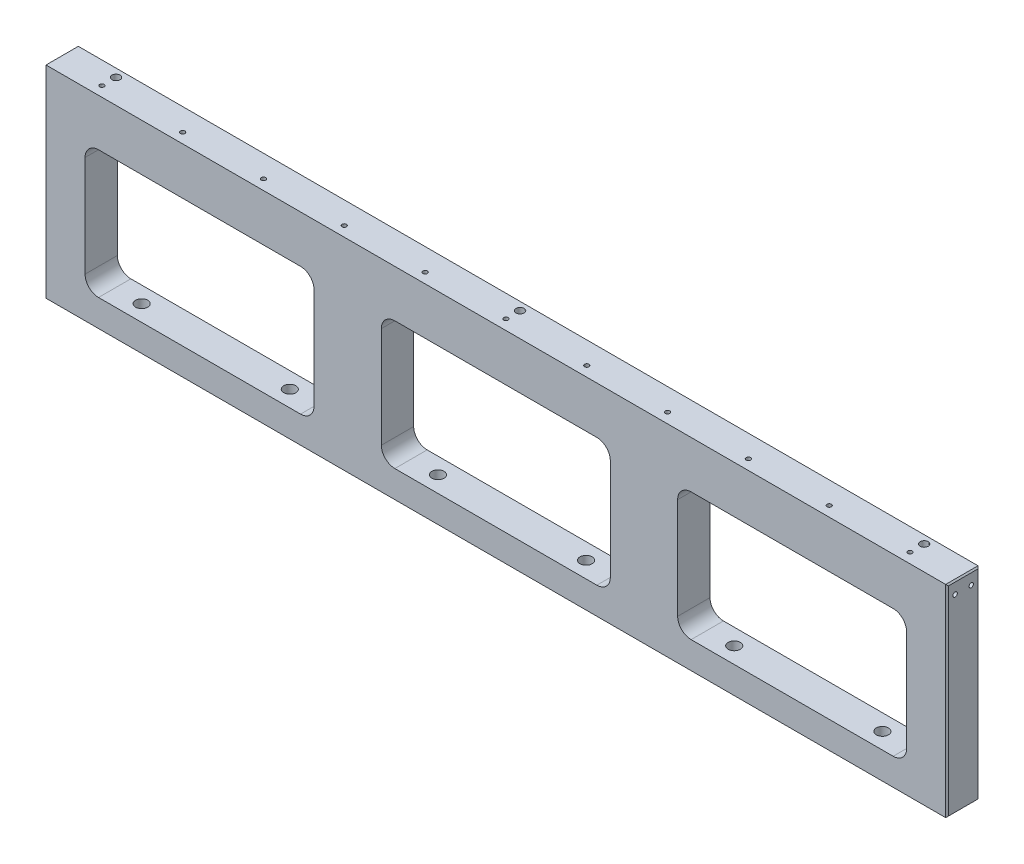
from build123d import *

# Parameters (mm, degrees)
SKETCH1_W                     = 670
SKETCH1_H                     = 150
BOSS_EXTRUDE1_DEPTH           = 12
CUT_EXTRUDE1_DEPTH            = 345.13078909
M8_CLEARANCE_HOLE1_D          = 9
M8_CLEARANCE_HOLE1_DEPTH      = 20
M4_TAPPED_HOLE1_D             = 3.3
M4_TAPPED_HOLE1_DEPTH         = 10.1
M4_TAPPED_HOLE1_TIP           = 0.991420021
SIZE_MM_BLIND_PIN_HOLE1_D     = 6
SIZE_MM_BLIND_PIN_HOLE1_DEPTH = 10.1
SIZE_MM_BLIND_PIN_HOLE1_TIP   = 1.802581857
CHAMFER1_SIZE                 = 1
M4_TAPPED_HOLE2_D             = 3.3
M4_TAPPED_HOLE2_DEPTH         = 10.1
M4_TAPPED_HOLE2_TIP           = 0.991420021
M4_TAPPED_HOLE3_D             = 3.3
M4_TAPPED_HOLE3_DEPTH         = 10.1
M4_TAPPED_HOLE3_TIP           = 0.991420021
M3_TAPPED_HOLE1_D             = 2.5
M3_TAPPED_HOLE1_DEPTH         = 7.5
M3_TAPPED_HOLE1_TIP           = 0.751075774
M4_TAPPED_HOLE4_D             = 3.3
M4_TAPPED_HOLE4_DEPTH         = 10.1
M4_TAPPED_HOLE4_TIP           = 0.991420021


with BuildPart() as part:
    # Sketch1 → Boss-Extrude1 (new, symmetric)
    with BuildSketch(Plane.XY):
        Rectangle(SKETCH1_W, SKETCH1_H)
    extrude(amount=BOSS_EXTRUDE1_DEPTH, both=True)

    # Sketch2 → Cut-Extrude1 (cut, through all)
    with BuildSketch(Plane.XY.offset(12)):
        with BuildLine():
            Line((-295, 40), (-145, 40))
            ThreePointArc((-145, 40), (-137.928932188, 37.071067812), (-135, 30))
            Line((-135, 30), (-135, -45))
            ThreePointArc((-135, -45), (-137.928932188, -52.071067812), (-145, -55))
            Line((-145, -55), (-295, -55))
            ThreePointArc((-295, -55), (-302.071067812, -52.071067812), (-305, -45))
            Line((-305, -45), (-305, 30))
            ThreePointArc((-305, 30), (-302.071067812, 37.071067812), (-295, 40))
        make_face()
        with BuildLine():
            Line((-75, 40), (75, 40))
            ThreePointArc((75, 40), (82.071067812, 37.071067812), (85, 30))
            Line((85, 30), (85, -45))
            ThreePointArc((85, -45), (82.071067812, -52.071067812), (75, -55))
            Line((75, -55), (-75, -55))
            ThreePointArc((-75, -55), (-82.071067812, -52.071067812), (-85, -45))
            Line((-85, -45), (-85, 30))
            ThreePointArc((-85, 30), (-82.071067812, 37.071067812), (-75, 40))
        make_face()
        with BuildLine():
            Line((145, 40), (295, 40))
            ThreePointArc((295, 40), (302.071067812, 37.071067812), (305, 30))
            Line((305, 30), (305, -45))
            ThreePointArc((305, -45), (302.071067812, -52.071067812), (295, -55))
            Line((295, -55), (145, -55))
            ThreePointArc((145, -55), (137.928932188, -52.071067812), (135, -45))
            Line((135, -45), (135, 30))
            ThreePointArc((135, 30), (137.928932188, 37.071067812), (145, 40))
        make_face()
    extrude(amount=-CUT_EXTRUDE1_DEPTH, mode=Mode.SUBTRACT)

    # M8 Clearance Hole1
    with Locations(Plane(origin=(0, -75, 0), x_dir=(-1, 0, 0), z_dir=(0, -1, 0))):
        with Locations((-275, 0), (275, 0), (165, 0), (55, 0), (-55, 0), (-165, 0)):
            Hole(M8_CLEARANCE_HOLE1_D / 2, depth=M8_CLEARANCE_HOLE1_DEPTH)

    # M4 Tapped Hole1
    with Locations(Plane(origin=(0, 75, 0), x_dir=(1, 0, 0), z_dir=(0, 1, 0))):
        with Locations((-300, -4.5), (-240, -4.5), (-180, -4.5), (-120, -4.5), (-60, -4.5), (0, -4.5), (60, -4.5), (120, -4.5), (180, -4.5), (240, -4.5), (300, -4.5)):
            Hole(M4_TAPPED_HOLE1_D / 2, depth=M4_TAPPED_HOLE1_DEPTH)
            with Locations((0, 0, -(M4_TAPPED_HOLE1_DEPTH + M4_TAPPED_HOLE1_TIP / 2))):  # 118° drill point
                Cone(0, M4_TAPPED_HOLE1_D / 2, M4_TAPPED_HOLE1_TIP, mode=Mode.SUBTRACT)

    # Size mm Blind Pin Hole1
    with Locations(Plane(origin=(0, 75, 0), x_dir=(1, 0, 0), z_dir=(0, 1, 0))):
        with Locations((300, 6), (-300, 6), (0, 6)):
            Hole(SIZE_MM_BLIND_PIN_HOLE1_D / 2, depth=SIZE_MM_BLIND_PIN_HOLE1_DEPTH)
            with Locations((0, 0, -(SIZE_MM_BLIND_PIN_HOLE1_DEPTH + SIZE_MM_BLIND_PIN_HOLE1_TIP / 2))):  # 118° drill point
                Cone(0, SIZE_MM_BLIND_PIN_HOLE1_D / 2, SIZE_MM_BLIND_PIN_HOLE1_TIP, mode=Mode.SUBTRACT)

    # Chamfer1
    chamfer1_edges = [part.edges().sort_by_distance(p)[0] for p in [
        (-335, 0, 12),
        (335, 0, 12),
        (-335, 0, -12),
        (335, 0, -12),
        (335, -75, 0),
        (-335, -75, 0),
        (-335, 75, 0),
        (335, 75, 0),
    ]]
    chamfer(chamfer1_edges, length=CHAMFER1_SIZE)

    # M4 Tapped Hole2
    with Locations(Plane(origin=(335, 0, 0), x_dir=(0, 0, -1), z_dir=(1, 0, 0))):
        with Locations((6, 66), (-6, 66)):
            Hole(M4_TAPPED_HOLE2_D / 2, depth=M4_TAPPED_HOLE2_DEPTH)
            with Locations((0, 0, -(M4_TAPPED_HOLE2_DEPTH + M4_TAPPED_HOLE2_TIP / 2))):  # 118° drill point
                Cone(0, M4_TAPPED_HOLE2_D / 2, M4_TAPPED_HOLE2_TIP, mode=Mode.SUBTRACT)

    # M4 Tapped Hole3
    with Locations(Plane.ZY.offset(335)):
        with Locations((-6, 66), (6, 66)):
            Hole(M4_TAPPED_HOLE3_D / 2, depth=M4_TAPPED_HOLE3_DEPTH)
            with Locations((0, 0, -(M4_TAPPED_HOLE3_DEPTH + M4_TAPPED_HOLE3_TIP / 2))):  # 118° drill point
                Cone(0, M4_TAPPED_HOLE3_D / 2, M4_TAPPED_HOLE3_TIP, mode=Mode.SUBTRACT)

    # M3 Tapped Hole1
    with Locations(Plane(origin=(0, 0, -12), x_dir=(1, 0, 0), z_dir=(0, 0, -1))):
        with Locations((314.85, -59), (-314.85, -59), (-295.15, -59), (295.15, -59)):
            Hole(M3_TAPPED_HOLE1_D / 2, depth=M3_TAPPED_HOLE1_DEPTH)
            with Locations((0, 0, -(M3_TAPPED_HOLE1_DEPTH + M3_TAPPED_HOLE1_TIP / 2))):  # 118° drill point
                Cone(0, M3_TAPPED_HOLE1_D / 2, M3_TAPPED_HOLE1_TIP, mode=Mode.SUBTRACT)

    # M4 Tapped Hole4
    with Locations(Plane(origin=(0, 0, -12), x_dir=(-1, 0, 0), z_dir=(0, 0, -1))):
        with Locations((109, 62.5), (109, 47.5)):
            Hole(M4_TAPPED_HOLE4_D / 2, depth=M4_TAPPED_HOLE4_DEPTH)
            with Locations((0, 0, -(M4_TAPPED_HOLE4_DEPTH + M4_TAPPED_HOLE4_TIP / 2))):  # 118° drill point
                Cone(0, M4_TAPPED_HOLE4_D / 2, M4_TAPPED_HOLE4_TIP, mode=Mode.SUBTRACT)


solid = part.part
